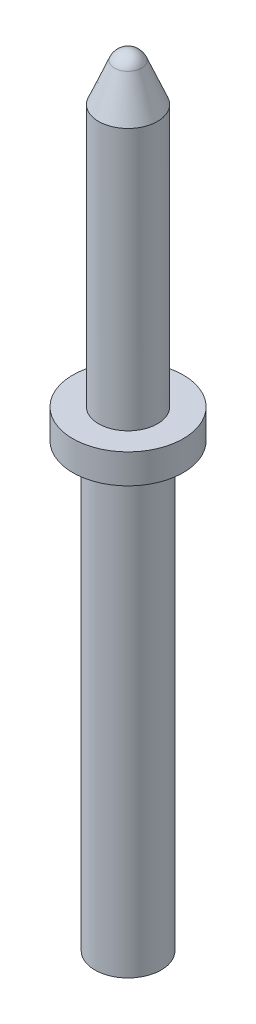
from build123d import *

# Parameters (mm, degrees)
SKETCH1_R           = 2.5
BOSS_EXTRUDE1_DEPTH = 20
SKETCH2_R           = 3.75
BOSS_EXTRUDE2_DEPTH = 2
SKETCH3_R           = 2.25
BOSS_EXTRUDE3_DEPTH = 30
SKETCH7_R           = 4
SKETCH7_R_2         = 2
CUT_EXTRUDE1_DEPTH  = 33.436476381


with BuildPart() as part:
    # Sketch1 → Boss-Extrude1 (new body)
    with BuildSketch(Plane(origin=(0, 0, 0), x_dir=(1, 0, 0), z_dir=(0, 1, 0))):
        with Locations(Location((0, 0, 0), (0, 0, 270))):
            Circle(SKETCH1_R)
    extrude(amount=BOSS_EXTRUDE1_DEPTH)

    # Sketch2 → Boss-Extrude2 (add)
    with BuildSketch(Plane.XZ):
        with Locations(Location((0, 0, 0), (0, 0, 270))):
            Circle(SKETCH2_R)
    extrude(amount=BOSS_EXTRUDE2_DEPTH)

    # Sketch3 → Boss-Extrude3 (add)
    with BuildSketch(Plane.XZ.offset(2)):
        with Locations(Location((0, 0, 0), (0, 0, 270))):
            Circle(SKETCH3_R)
    extrude(amount=BOSS_EXTRUDE3_DEPTH)

    # Sketch4 → Revolve1 (revolve)
    with BuildSketch(Plane.XY, mode=Mode.PRIVATE) as revolve1_sk:
        with BuildLine():
            Line((1, 20), (0, 20))
            Line((0, 20), (0, 21))
            ThreePointArc((0, 21), (0.707106781, 20.707106781), (1, 20))
        make_face()
    revolve(revolve1_sk.sketch.rotate(Axis((0, 20, 0), (0, 1, 0)), 90), axis=Axis((0, 20, 0), (0, 1, 0)))

    # Sketch5 → Cut-Revolve1 (revolve, cut)
    with BuildSketch(Plane(origin=(0, 0, 0), x_dir=(0, 0, -1), z_dir=(1, 0, 0)), mode=Mode.PRIVATE) as cut_revolve1_sk:
        Polygon((1.0823922, 20), (2.5, 16.577592024), (2.5, 20), align=None)
    revolve(cut_revolve1_sk.sketch.rotate(Axis((0, 15, 0), (0, -1, 0)), 90), axis=Axis((0, 15, 0), (0, -1, 0)), mode=Mode.SUBTRACT)

    # Sketch6 → Revolve2 (revolve)
    with BuildSketch(Plane(origin=(0, 0, 0), x_dir=(0, 0, -1), z_dir=(1, 0, 0))):
        with BuildLine():
            Line((1.0823922, 20), (0.923879533, 20.382683432))
            ThreePointArc((0.923879533, 20.382683432), (0.98078528, 20.195090322), (1, 20))
            Line((1, 20), (1.0823922, 20))
        make_face()
    revolve(axis=Axis((0, 16, 0), (0, 1, 0)))

    # Sketch7 → Cut-Extrude1 (cut, through all)
    with BuildSketch(Plane(origin=(0, 0, 0), x_dir=(1, 0, 0), z_dir=(0, 1, 0))):
        Circle(SKETCH7_R)
        with Locations(Location((0, 0, 0), (0, 0, 90))):
            Circle(SKETCH7_R_2, mode=Mode.SUBTRACT)
    extrude(amount=CUT_EXTRUDE1_DEPTH, mode=Mode.SUBTRACT)


solid = part.part
